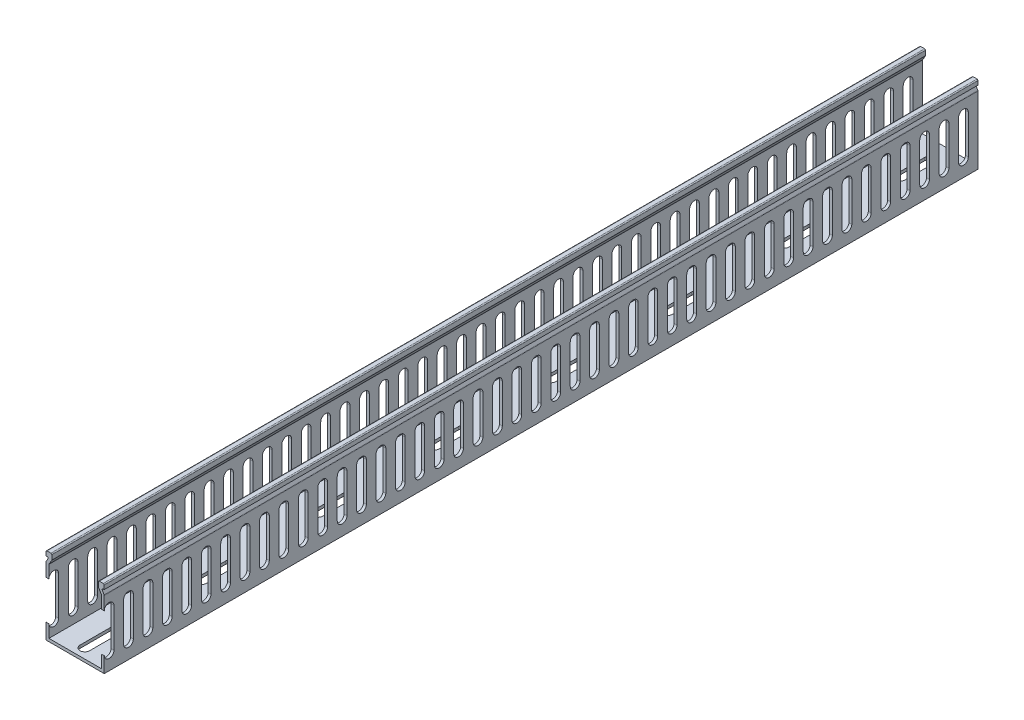
from build123d import *

# Parameters (mm, degrees)
EXTRUDE_1_DEPTH        = 450
CUT_EXTRUDE_2_DEPTH    = 453.769256907
PATTERN_LINEAR_1_COUNT = 130
PATTERN_LINEAR_1_PITCH = 10
CUT_EXTRUDE_3_DEPTH    = 453.023229492
PATTERN_LINEAR_2_COUNT = 25
PATTERN_LINEAR_2_PITCH = 60


with BuildPart() as part:
    # 草圖1 → 伸長1 (new body)
    with BuildSketch(Plane.XY):
        with BuildLine():
            Line((14.928746463, 35.118755895), (13.954348727, 36.742752122))
            ThreePointArc((13.954348727, 36.742752122), (13.947995236, 37.246349407), (14.383095189, 37.5))
            Line((14.383095189, 37.5), (15, 37.5))
            Line((15, 37.5), (15, 39.5))
            ThreePointArc((15, 39.5), (14.853553391, 39.853553391), (14.5, 40))
            Line((14.5, 40), (12.5, 40))
            ThreePointArc((12.5, 40), (12.146446609, 39.853553391), (12, 39.5))
            Line((12, 39.5), (12, 37.223016035))
            ThreePointArc((12, 37.223016035), (12.018142536, 37.089549244), (12.071253537, 36.965768157))
            Line((12.071253537, 36.965768157), (13.428746463, 34.703279948))
            ThreePointArc((13.428746463, 34.703279948), (13.481857464, 34.579498861), (13.5, 34.44603207))
            Line((13.5, 34.44603207), (13.5, 1.5))
            Line((13.5, 1.5), (-13.5, 1.5))
            Line((-13.5, 1.5), (-13.5, 34.44603207))
            ThreePointArc((-13.5, 34.44603207), (-13.481857464, 34.579498861), (-13.428746463, 34.703279948))
            Line((-13.428746463, 34.703279948), (-12.071253537, 36.965768157))
            ThreePointArc((-12.071253537, 36.965768157), (-12.018142536, 37.089549244), (-12, 37.223016035))
            Line((-12, 37.223016035), (-12, 39.5))
            ThreePointArc((-12, 39.5), (-12.146446609, 39.853553391), (-12.5, 40))
            Line((-12.5, 40), (-14.5, 40))
            ThreePointArc((-14.5, 40), (-14.853553391, 39.853553391), (-15, 39.5))
            Line((-15, 39.5), (-15, 37.5))
            Line((-15, 37.5), (-14.383095189, 37.5))
            ThreePointArc((-14.383095189, 37.5), (-13.947995236, 37.246349407), (-13.954348727, 36.742752122))
            Line((-13.954348727, 36.742752122), (-14.928746463, 35.118755895))
            ThreePointArc((-14.928746463, 35.118755895), (-14.981857464, 34.994974808), (-15, 34.861508018))
            Line((-15, 34.861508018), (-15, 0))
            Line((-15, 0), (15, 0))
            Line((15, 0), (15, 34.861508018))
            ThreePointArc((15, 34.861508018), (14.981857464, 34.994974808), (14.928746463, 35.118755895))
        make_face()
    extrude(amount=EXTRUDE_1_DEPTH)

    # 草圖2 → 伸長2 (cut, through all)
    with BuildSketch(Plane.ZY.offset(15)):
        with BuildLine():
            Line((5, 28), (5, 8))
            ThreePointArc((5, 8), (7.5, 5.5), (10, 8))
            Line((10, 8), (10, 28))
            ThreePointArc((10, 28), (7.5, 30.5), (5, 28))
        make_face()
    cut_extrude_2 = extrude(amount=-CUT_EXTRUDE_2_DEPTH, mode=Mode.SUBTRACT)

    # 直線複製排列1: 伸長2 ×130
    with Locations(*[(0, 0, i * PATTERN_LINEAR_1_PITCH) for i in range(1, PATTERN_LINEAR_1_COUNT)]):
        add(cut_extrude_2, mode=Mode.SUBTRACT)

    # 草圖3 → 伸長3 (cut, through all)
    with BuildSketch(Plane.XZ):
        with BuildLine():
            Line((-2.5, 25), (-2.5, 10))
            ThreePointArc((-2.5, 10), (0, 7.5), (2.5, 10))
            Line((2.5, 10), (2.5, 25))
            ThreePointArc((2.5, 25), (0, 27.5), (-2.5, 25))
        make_face()
    cut_extrude_3 = extrude(amount=-CUT_EXTRUDE_3_DEPTH, mode=Mode.SUBTRACT)

    # 直線複製排列2: 伸長3 ×25
    with Locations(*[(0, 0, i * PATTERN_LINEAR_2_PITCH) for i in range(1, PATTERN_LINEAR_2_COUNT)]):
        add(cut_extrude_3, mode=Mode.SUBTRACT)


solid = part.part
